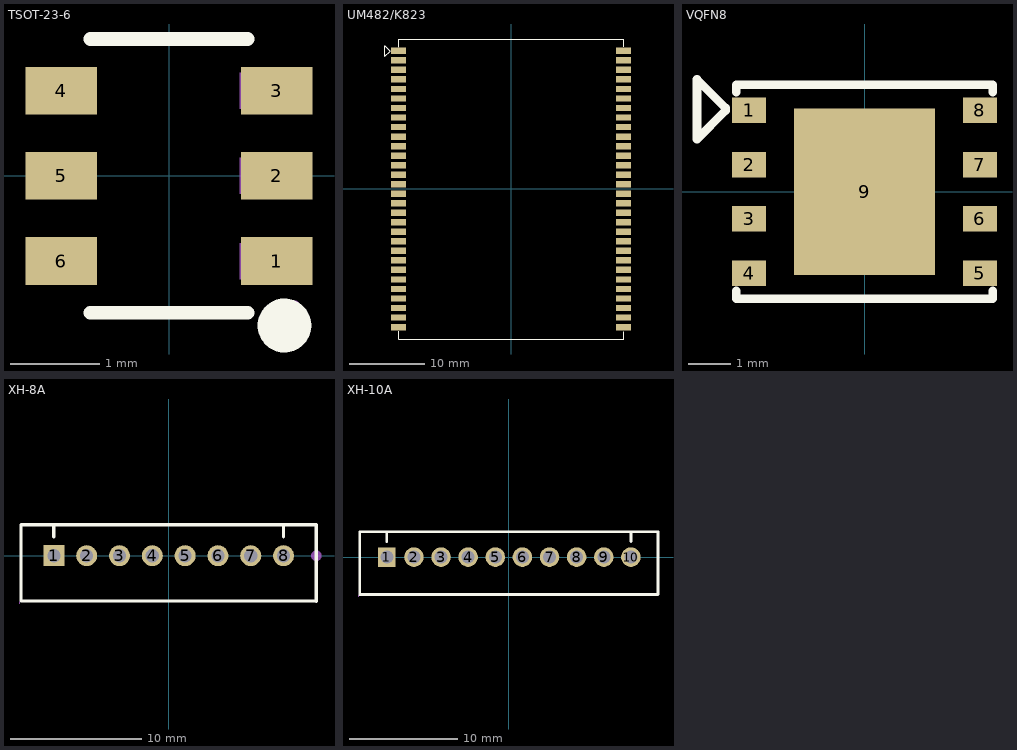
[diagram p0: the footprints below, top view; thin cyan lines are the x and y axes]
# Altium footprint library MISC84456-2.PcbLib: 53 footprints (part 4 of 4)
Each footprint in its own frame and in the unit in brackets; x right, y up, seen from the top. Pads: shape width x height; smd on the part's side, far side on the other; paste and mask are expansions set on the pad; w line width, h text height; cw(c..) or ccw(c..) is an arc to the next point about the centre after c.

## TSOT-23-6 [mm]
pads (6):
  rect 0.8x0.532 smd: 1(1.2,-0.95) 2(1.2,0) 3(1.2,0.95) 4(-1.2,0.95) 5(-1.2,0) 6(-1.2,-0.95)
Top Overlay:
  circle w0.3: c1.288,-1.669 r0.15
  lines w0.152: -0.876,-1.526 0.876,-1.526 ; -0.876,1.526 0.876,1.526
Mechanical 5:
  pour cut-out: 0.79,0.75 0.79,1.15 0.96,1.15 0.96,0.75
  pour cut-out: 0.79,-0.2 0.79,0.2 0.96,0.2 0.96,-0.2
  pour cut-out: 0.79,-1.15 0.79,-0.75 0.96,-0.75 0.96,-1.15
Mechanical 6:
  circle w0.06: c1.4,-1.45 r0.03

## UM482/K823 [mm]
pads (60):
  rect 2.01x0.85 smd: 1(-15,18.415) 2(-15,17.145) 3(-15,15.875) 4(-15,14.605) 5(-15,13.335) 6(-15,12.065) 7(-15,10.795) 8(-15,9.525) 9(-15,8.255) 10(-15,6.985) 11(-15,5.715) 12(-15,4.445) 13(-15,3.175) 14(-15,1.905) 15(-15,0.635) 16(-15,-0.635) 17(-15,-1.905) 18(-15,-3.175) 19(-15,-4.445) 20(-15,-5.715) 21(-15,-6.985) 22(-15,-8.255) 23(-15,-9.525) 24(-15,-10.795) 25(-15,-12.065) 26(-15,-13.335) 27(-15,-14.605) 28(-15,-15.875) 29(-15,-17.145) 30(-15,-18.415) 31(15,-18.415) 32(15,-17.145) 33(15,-15.875) 34(15,-14.605) 35(15,-13.335) 36(15,-12.065) 37(15,-10.795) 38(15,-9.525) 39(15,-8.255) 40(15,-6.985) 41(15,-5.715) 42(15,-4.445) 43(15,-3.175) 44(15,-1.905) 45(15,-0.635) 46(15,0.635) 47(15,1.905) 48(15,3.175) 49(15,4.445) 50(15,5.715) 51(15,6.985) 52(15,8.255) 53(15,9.525) 54(15,10.795) 55(15,12.065) 56(15,13.335) 57(15,14.605) 58(15,15.875) 59(15,17.145) 60(15,18.415)
Top Overlay:
  lines w0.1: -15,-18.95 -15,-20.005 15,-20.005 15,-19.01 ; -15,18.92 -15,19.995 15,19.995 15,18.93 ; -16.81,17.69 -16.81,19.11 -16.14,18.44 -16.13,18.44 -16.13,18.37 -16.81,17.69

## VQFN8 [mm]
pads (9):
  rect 0.8x0.6 smd: 1(-2.7,1.905) 2(-2.7,0.635) 3(-2.7,-0.635) 4(-2.7,-1.905) 5(2.7,-1.905) 6(2.7,-0.635) 7(2.7,0.635) 8(2.7,1.905)
  rect 3.3x3.9 smd: 9(0,0)
Top Overlay:
  lines w0.2: -3.25,1.95 -3.25,1.96 ; -3,-2.32 -3,-2.5 3,-2.5 3,-2.32 ; -3,2.33 -3,2.5 3,2.5 3,2.33 ; -3.25,1.96 -3.25,1.9 -3.92,1.23 -3.92,2.63 -3.25,1.96

## XH-8A [mm]
pads (8):
  rect 1.6x1.6 hole 1: 1(-8.75,0)
  round 1.6 hole 1: 2(-6.25,0) 3(-3.75,0) 4(-1.25,0) 5(1.25,0) 6(3.75,0) 7(6.25,0) 8(8.75,0)
Top Overlay:
  lines w0.254: -8.75,1.45 -8.75,2.35 ; 8.74,1.44 8.74,2.339 ; 11.24,-3.46 11.24,2.34 ; 11.25,-3.45 -11.25,-3.45 -11.25,2.35 11.25,2.35
Mechanical 5:
  circle w0.4: c11.25,0 r0.2
  circle w0.4: c8.75,0 r0.2
  circle w0.4: c6.25,0 r0.2
  circle w0.4: c3.75,0 r0.2
  circle w0.4: c1.25,0 r0.2
  circle w0.4: c-1.25,0 r0.2
  circle w0.4: c-3.75,0 r0.2
  circle w0.4: c-6.25,0 r0.2
  circle w0.4: c-8.75,0 r0.2
Mechanical 6:
  circle w0.06: c-11.377,-3.577 r0.03

## XH-10A [mm]
pads (10):
  rect 1.6x1.8 hole 1.2: 1(-11.25,0)
  round 1.8 hole 1.2: 2(-8.75,0) 3(-6.25,0) 4(-3.75,0) 5(-1.25,0) 6(1.25,0) 7(3.75,0) 8(6.25,0) 9(8.75,0) 10(11.25,0)
Top Overlay:
  lines w0.254: -11.25,1.45 -11.25,2.35 ; 11.25,1.45 11.25,2.35 ; -13.75,-3.45 13.75,-3.45 13.75,2.35 -13.75,2.35 -13.75,-3.45
Mechanical 5:
  circle w0.5: c-11.25,0 r0.25
  circle w0.5: c-8.75,0 r0.25
  circle w0.5: c-6.25,0 r0.25
  circle w0.5: c-3.75,0 r0.25
  circle w0.5: c-1.25,0 r0.25
  circle w0.5: c1.25,0 r0.25
  circle w0.5: c3.75,0 r0.25
  circle w0.5: c6.25,0 r0.25
  circle w0.5: c8.75,0 r0.25
  circle w0.5: c11.25,0 r0.25
Mechanical 6:
  circle w0.06: c-13.877,-3.577 r0.03